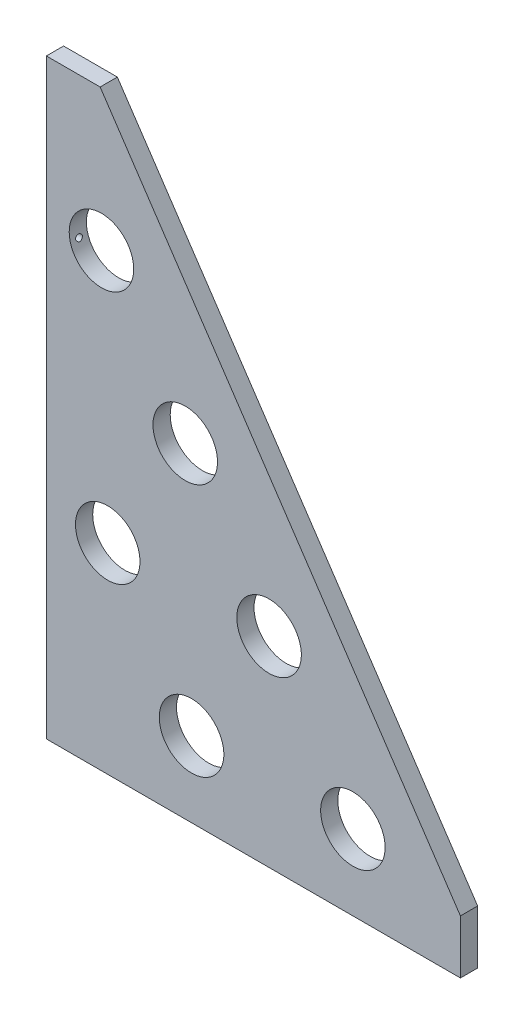
SolidWorks part; units mm, degrees
material "6061-T4 (SS)"
ref_plane "前视基准面" through (0, 0, 0) normal (0, 0, 1) x (1, 0, 0)
ref_plane "上视基准面" through (0, 0, 0) normal (0, 1, 0) x (1, 0, 0)
ref_plane "右视基准面" through (0, 0, 0) normal (1, 0, 0) x (0, 0, -1)
sketch "草图1" plane through (0, 0, 0) normal (0, 0, 1) x (1, 0, 0)
  line L0 (0, 0) -> (385, 0)
  line L1 (0, 0) -> (0, 550)
  line L2 (0, 550) -> (50, 550)
  line L3 (50, 550) -> (385, 50)
  line L4 (385, 0) -> (385, 50)
  dimension "D1" = 550
  dimension "D2" = 385
  dimension "D3" = 50
  dimension "D4" = 50
extrude "凸台-拉伸1" add sketch "草图1" along normal mid plane 16
hole_wizard "M8 螺纹孔1" positions "草图2" profile "草图3" tap size "M8" standard "GB"
sketch "草图2" plane through (0, 0, 0) normal (-1, 0, 0) x (0, 0, 1)
  line L0 (0, 550) -> (0, 0) construction
  line L1 (8, 550) -> (-8, 550) construction
  point P6 (0, 520)
  dimension "D1" = 30
sketch "草图3" plane through (0, 520, 0) normal (0, 1, 0) x (0, 0, 1)
  line L0 (0, 0) -> (0, 24.2929)
  line L1 (0, 24.2929) -> (3.4, 22.25)
  line L2 (3.4, 22.25) -> (3.4, 0)
  line L5 (3.4, 0) -> (0, 0)
  line L10 (0, 24.2929) -> (-3.4, 22.25) construction
  line L11 (0, -6.35) -> (0, 107.95) construction
  dimension "螺纹孔钻头直径" = 6.8
  dimension "螺纹孔钻头深度" = 22.25
  dimension "导头角度" = 118
cosmetic thread "孔螺蚊线2" parameters "D1"=16, "D2"=8
pattern_linear "阵列(线性)1" count 10 spacing 55 along (0, -1, 0) of "M8 螺纹孔1"
hole_wizard "M8 螺纹孔2" positions "草图4" profile "草图5" tap size "M8" standard "GB"
sketch "草图4" plane through (0, 0, 0) normal (0, -1, 0) x (-1, 0, 0)
  line L0 (-385, 0) -> (0, 0) construction
  line L1 (-385, -8) -> (-385, 8) construction
  point P7 (-20, 0)
  dimension "D1" = 20
sketch "草图5" plane through (20, 0, 0) normal (1, 0, 0) x (0, 0, -1)
  line L0 (0, 0) -> (0, 24.2929)
  line L1 (0, 24.2929) -> (3.4, 22.25)
  line L2 (3.4, 22.25) -> (3.4, 0)
  line L5 (3.4, 0) -> (0, 0)
  line L10 (0, 24.2929) -> (-3.4, 22.25) construction
  line L11 (0, -6.35) -> (0, 107.95) construction
  dimension "螺纹孔钻头直径" = 6.8
  dimension "螺纹孔钻头深度" = 22.25
  dimension "导头角度" = 118
cosmetic thread "孔螺蚊线1" parameters "D1"=16, "D2"=8
pattern_linear "阵列(线性)2" count 8 spacing 50 along (1, 0, 0) of "M8 螺纹孔2"
sketch "草图6" plane through (0, 0, -8) normal (0, 0, -1) x (-1, 0, 0)
  line L0 (0, 550) -> (0, 0) construction
  line L1 (0, 0) -> (-385, 0) construction
  line L2 (-285, 70) -> (-129.1476, 302.6156) construction
  line L3 (-129.1476, 302.6156) -> (-51.2213, 418.9234) construction
  line L4 (-135, 70) -> (-57.0738, 186.3078) construction
  line L5 (-385, 50) -> (-50, 550) construction
  line L6 (-285, 70) -> (-135, 70) construction
  circle A0 centre (-285, 70) radius 30
  circle A1 centre (-129.1476, 302.6156) radius 30
  circle A2 centre (-207.0738, 186.3078) radius 30
  circle A3 centre (-135, 70) radius 30
  circle A4 centre (-51.2213, 418.9234) radius 30
  circle A5 centre (-57.0738, 186.3078) radius 30
  dimension "D1" = 60
  dimension "D2" = 285
  dimension "D3" = 70
  dimension "D4" = 280
  dimension "D5" = 150
  dimension "D6" = 140
  dimension "D7" = 140
extrude "切除-拉伸1" cut sketch "草图6" against normal through all
